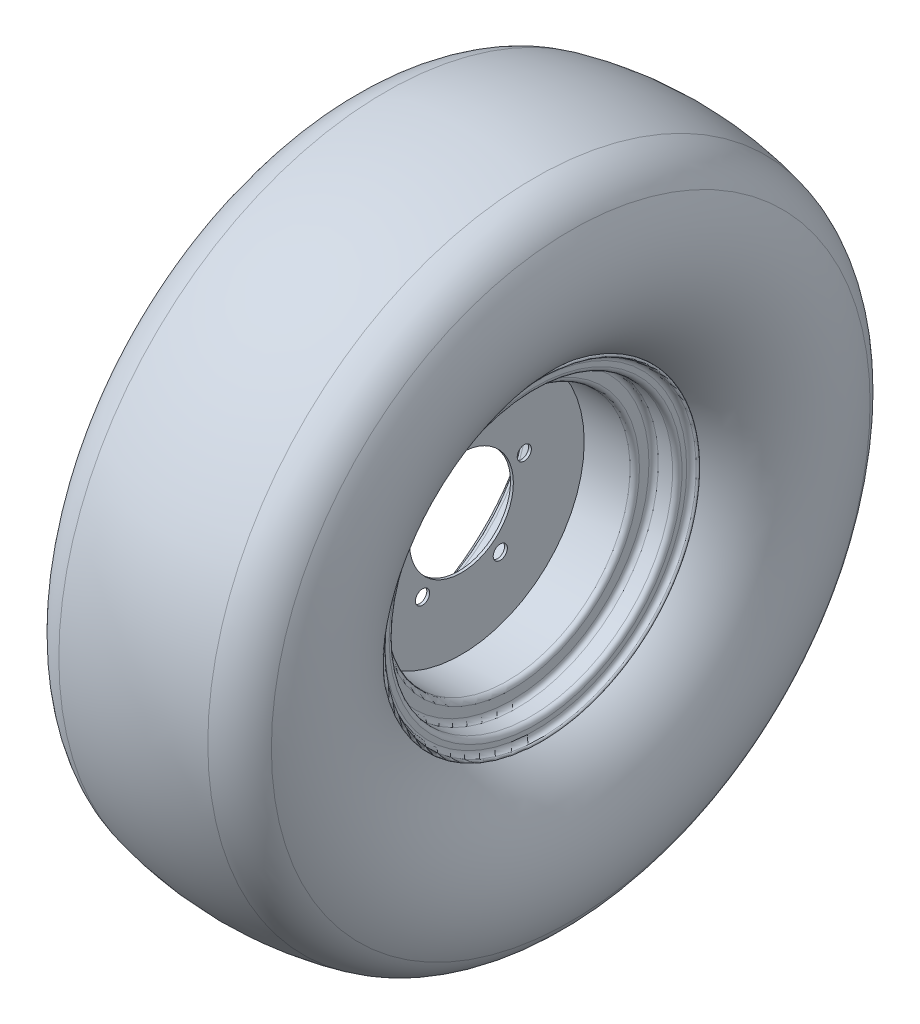
SolidWorks part; units mm, degrees
ref_plane "前视基准面" through (0, 0, 0) normal (0, 0, 1) x (1, 0, 0)
ref_plane "上视基准面" through (0, 0, 0) normal (0, 1, 0) x (1, 0, 0)
ref_plane "右视基准面" through (0, 0, 0) normal (1, 0, 0) x (0, 0, -1)
sketch "草图1" plane through (0, 0, 0) normal (0, 0, 1) x (1, 0, 0)
  line L0 (-50, 0) -> (50, 0)
  line L1 (55, -5) -> (55, -15)
  line L2 (60, -20) -> (75, -20)
  line L3 (80, -25) -> (80, -30)
  line L4 (0, 0) -> (0, -35) construction
  line L5 (-80, -25) -> (-80, -30)
  line L6 (-60, -20) -> (-75, -20)
  line L7 (-55, -5) -> (-55, -15)
  line L8 (-77, -25) -> (-77, -30)
  line L9 (-60, -23) -> (-75, -23)
  line L10 (-52, -5) -> (-52, -15)
  line L11 (-50, -3) -> (50, -3)
  line L12 (52, -5) -> (52, -15)
  line L13 (60, -23) -> (75, -23)
  line L14 (77, -25) -> (77, -30)
  line L15 (-65.4049, 130) -> (165.0532, 130) construction
  arc A0 (80, -30) -> (85, -35) centre (85, -30) ccw
  arc A1 (75, -20) -> (80, -25) centre (75, -25) cw
  arc A2 (55, -15) -> (60, -20) centre (60, -15) ccw
  arc A3 (50, 0) -> (55, -5) centre (50, -5) cw
  arc A4 (-50, 0) -> (-55, -5) centre (-50, -5) ccw
  arc A5 (-55, -15) -> (-60, -20) centre (-60, -15) cw
  arc A6 (-75, -20) -> (-80, -25) centre (-75, -25) ccw
  arc A7 (-80, -30) -> (-85, -35) centre (-85, -30) cw
  arc A8 (-77, -30) -> (-85, -38) centre (-85, -30) cw
  arc A9 (-75, -23) -> (-77, -25) centre (-75, -25) ccw
  arc A10 (-52, -15) -> (-60, -23) centre (-60, -15) cw
  arc A11 (-50, -3) -> (-52, -5) centre (-50, -5) ccw
  arc A12 (50, -3) -> (52, -5) centre (50, -5) cw
  arc A13 (52, -15) -> (60, -23) centre (60, -15) ccw
  arc A14 (75, -23) -> (77, -25) centre (75, -25) cw
  arc A15 (77, -30) -> (85, -38) centre (85, -30) ccw
  arc A16 (-85, -35) -> (-85, -38) centre (-85, -36.5) ccw
  arc A17 (85, -35) -> (85, -38) centre (85, -36.5) cw
  point P4 (0, 0)
  point P13 (80, -20)
  point P16 (55, -20)
  point P19 (55, 0)
  point P31 (-55, 0)
  point P32 (-55, -20)
  point P33 (-80, -20)
  dimension "D5" = 5
  dimension "D6" = 5
  dimension "D1" = 100
  dimension "D2" = 20
  dimension "D3" = 25
  dimension "D4" = 10
  dimension "D7" = 3
  dimension "D8" = 165
revolve "旋转1" add sketch "草图1" angle 360 about L15
sketch "草图2" plane through (0, 0, 0) normal (1, 0, 0) x (0, 0, -1)
  circle A0 centre (0, 130) radius 130
  circle A1 centre (0, 130) radius 55
  circle A3 centre (0, 200) radius 7.5
  circle A9 centre (0, 130) radius 70 construction
  circle A10 centre (66.574, 151.6312) radius 7.5
  circle A11 centre (41.145, 73.3688) radius 7.5
  circle A12 centre (-41.145, 73.3688) radius 7.5
  circle A13 centre (-66.574, 151.6312) radius 7.5
  dimension "D1" = 110
  dimension "D2" = 140
  dimension "D3" = 15
  dimension "D4" = 5
extrude "凸台-拉伸1" add sketch "草图2" along normal mid plane 3 separate body
sketch "草图3" plane through (0, 0, 0) normal (0, 0, 1) x (1, 0, 0)
  line L0 (-77, 285) -> (-77, 290)
  line L1 (-85, 298) -> (-85, -38) construction
  line L2 (50, 130) -> (-52, 130) construction
  line L5 (-75, 283) -> (-60, 283)
  line L6 (50, 263) -> (50, -3) construction
  line L9 (-52, 275) -> (-52, 265)
  line L11 (-50, 263) -> (50, 263)
  line L12 (52, 265) -> (52, 275)
  line L13 (60, 283) -> (75, 283)
  line L14 (77, 285) -> (77, 290)
  line L15 (-52, -5) -> (-52, 265) construction
  arc A0 (-77, 290) -> (-85, 298) centre (-85, 290) ccw
  arc A1 (-78.8329, 475.7579) -> (78.8329, 475.7579) centre (0, 144.1667) cw
  arc A2 (-85, 298) -> (-117.2174, 446.8581) centre (-17.3744, 390.5517) cw
  arc A3 (-117.2174, 446.8581) -> (-78.8329, 475.7579) centre (-64.9552, 417.3849) cw
  arc A4 (117.2174, 446.8581) -> (78.8329, 475.7579) centre (64.9552, 417.3849) ccw
  arc A5 (85, 298) -> (117.2174, 446.8581) centre (17.3744, 390.5517) ccw
  arc A6 (77, 290) -> (85, 298) centre (85, 290) cw
  arc A7 (-77, 285) -> (-75, 283) centre (-75, 285) ccw
  arc A8 (-60, 283) -> (-52, 275) centre (-60, 275) cw
  arc A9 (-52, 265) -> (-50, 263) centre (-50, 265) ccw
  arc A10 (-52, 265) -> (-50, 263) centre (-50, 265) ccw construction
  arc A11 (50, 263) -> (52, 265) centre (50, 265) ccw
  arc A12 (52, 275) -> (60, 283) centre (60, 275) cw
  arc A13 (75, 283) -> (77, 285) centre (75, 285) ccw
  point P25 (0, 485)
  dimension "D3" = 60
  dimension "D1" = 114.6256
  dimension "D2" = 340.8333
revolve "旋转2" add sketch "草图3" angle 360 about L2
